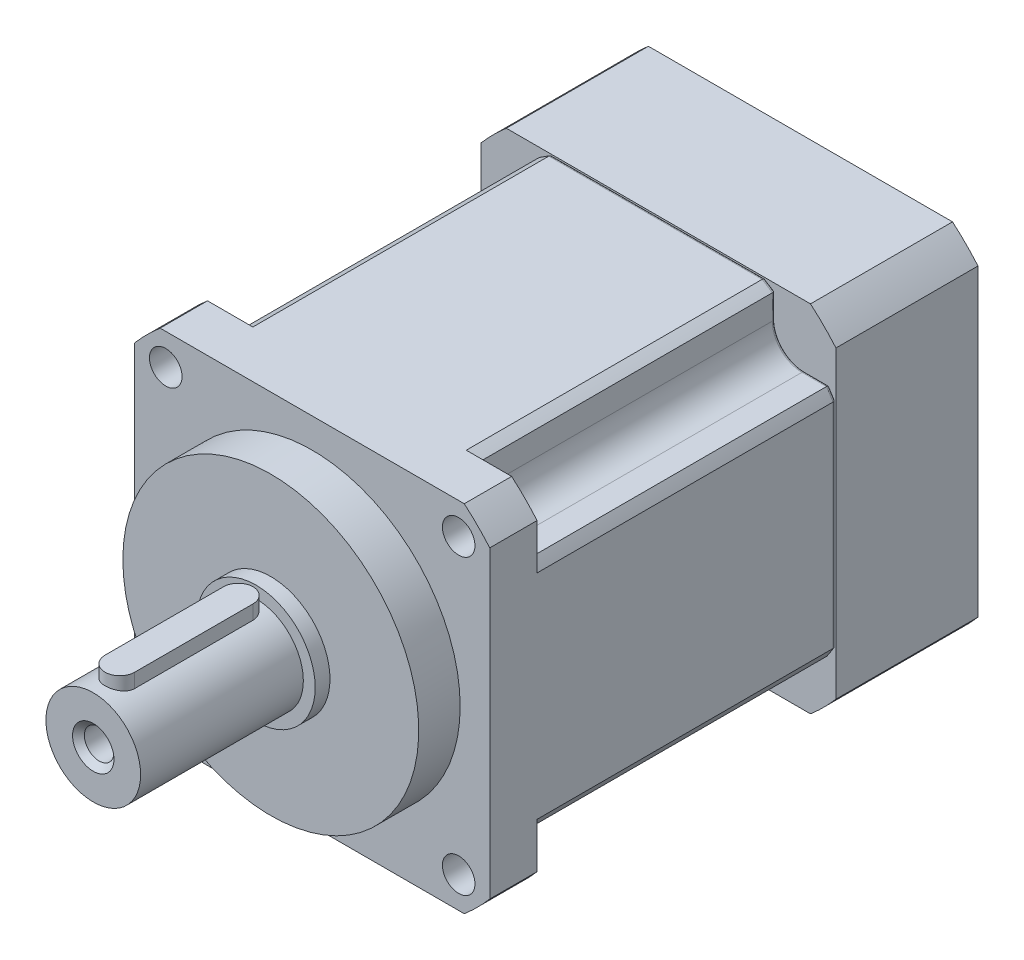
from build123d import *

# Parameters (mm, degrees)
SKETCH_1_R               = 25
EXTRUDE_2137_DEPTH       = 37
SKETCH_2_OUTSIDE_W       = 67.962
SKETCH_2_OUTSIDE_H       = 67.962
SKETCH_2_OUTSIDE_R       = 10
CUT_EXTRUDE_1_DEPTH      = 47.368092477
SKETCH_3_OUTSIDE_W       = 67.962
SKETCH_3_OUTSIDE_H       = 67.962
SKETCH_3_OUTSIDE_R       = 8
CUT_EXTRUDE_2_DEPTH      = 27.5
EXTRUDE_2_REACH          = 58.736
EXTRUDE_2_END_RADIUS     = 8
SKETCH_6_W               = 60
SKETCH_6_H               = 60
EXTRUDE_2668_DEPTH       = 58.5
CUT_EXTRUDE_8_DEPTH      = 66.956425009
PATTERN_CIRCULAR_2_COUNT = 4
CUT_EXTRUDE_6_REACH      = 74.265
SKETCH_9_R               = 2.75
PATTERN_CIRCULAR_1_COUNT = 4
SKETCH_10_OUTSIDE_W      = 87.55
SKETCH_10_OUTSIDE_H      = 87.55
SKETCH_10_OUTSIDE_R      = 39.5
CUT_EXTRUDE_7_DEPTH      = 73.265136823
FILLET_3_R               = 0.5
SKETCH_15_W              = 60
SKETCH_15_H              = 60
EXTRUDE_8537_DEPTH       = 24
SKETCH_21_OUTSIDE_W      = 91.312
SKETCH_21_OUTSIDE_H      = 91.312
SKETCH_21_OUTSIDE_R      = 39.5
CUT_EXTRUDE_10_DEPTH     = 24
SKETCH_22_R              = 25
CUT_EXTRUDE_11_DEPTH     = 5
SKETCH_30_R              = 7
CUT_EXTRUDE_15_DEPTH     = 32
PATTERN_CIRCULAR_3_COUNT = 4


with BuildPart() as part:
    # 草图1 → Extrude 2137 (new body)
    with BuildSketch(Plane.XY):
        Circle(SKETCH_1_R)
    extrude(amount=EXTRUDE_2137_DEPTH)

    # 草图2 outside → 切除-拉伸1 (cut, through all)
    with BuildSketch(Plane(origin=(0, 0, 7), x_dir=(-1, 0, 0), z_dir=(0, 0, -1))):
        Rectangle(SKETCH_2_OUTSIDE_W, SKETCH_2_OUTSIDE_H)
        Circle(SKETCH_2_OUTSIDE_R, mode=Mode.SUBTRACT)
    extrude(amount=-CUT_EXTRUDE_1_DEPTH, mode=Mode.SUBTRACT)

    # 草图3 outside → 切除-拉伸2 (cut)
    with BuildSketch(Plane.XY.offset(37)):
        Rectangle(SKETCH_3_OUTSIDE_W, SKETCH_3_OUTSIDE_H)
        Circle(SKETCH_3_OUTSIDE_R, mode=Mode.SUBTRACT)
    extrude(amount=-CUT_EXTRUDE_2_DEPTH, mode=Mode.SUBTRACT)

    # 凸台-拉伸2: up to this cylinder (the profile starts outside it)
    extrude_2_end = Plane(origin=(0, 0, 22.5), z_dir=(0, 0, 1)) * Cylinder(EXTRUDE_2_END_RADIUS, 134.472, mode=Mode.PRIVATE)
    # 草图4 → 凸台-拉伸2 (add, up to the surface)
    with BuildSketch(Plane(origin=(0, 10, 0), x_dir=(-1, 0, 0), z_dir=(0, 1, 0)), mode=Mode.PRIVATE) as extrude_2_sk1:
        with BuildLine():
            Line((-2.5, 32.5), (-2.5, 12.5))
            ThreePointArc((-2.5, 12.5), (0, 10), (2.5, 12.5))
            Line((2.5, 12.5), (2.5, 32.5))
            ThreePointArc((2.5, 32.5), (0, 35), (-2.5, 32.5))
        make_face()
    extrude_2_tool1 = extrude(extrude_2_sk1.sketch, amount=-EXTRUDE_2_REACH, mode=Mode.PRIVATE) - extrude_2_end
    add(extrude_2_tool1.solids().sort_by_distance((0, 10, 22.5))[0])

    # 草图6 → Extrude 2668 (add)
    with BuildSketch(Plane(origin=(0, 0, 0), x_dir=(-1, 0, 0), z_dir=(0, 0, -1))):
        Rectangle(SKETCH_6_W, SKETCH_6_H)
    extrude(amount=EXTRUDE_2668_DEPTH)

    # 草图7 → 切除-拉伸8 (cut, through all)
    with BuildSketch(Plane.XY.offset(-8)):
        with BuildLine():
            Line((24.748737342, 19.748737342), (28.896148072, 19.748737342))
            ThreePointArc((28.896148072, 19.748737342), (29.460643379, 18.896308944), (30, 18.027756377))
            Line((30, 18.027756377), (30, 30))
            Line((30, 30), (18.027756377, 30))
            ThreePointArc((18.027756377, 30), (18.896308944, 29.460643379), (19.748737342, 28.896148072))
            Line((19.748737342, 28.896148072), (19.748737342, 24.748737342))
            ThreePointArc((19.748737342, 24.748737342), (21.213203436, 21.213203436), (24.748737342, 19.748737342))
        make_face()
    cut_extrude_8 = extrude(amount=-CUT_EXTRUDE_8_DEPTH, mode=Mode.SUBTRACT)

    # 阵列(圆周)2: 切除-拉伸8 ×4 about axis
    pattern_circular_2_axis = Axis((0, 0, 0), (0, 0, 1))
    for i in range(1, PATTERN_CIRCULAR_2_COUNT):
        add(cut_extrude_8.rotate(pattern_circular_2_axis, i * 360 / PATTERN_CIRCULAR_2_COUNT), mode=Mode.SUBTRACT)

    # 草图9 → 切除-拉伸6 (cut, up to next)
    with BuildSketch(Plane.XY, mode=Mode.PRIVATE) as cut_extrude_6_sk1:
        with Locations((24.748737342, 24.748737342)):
            Circle(SKETCH_9_R)
    cut_extrude_6_tool1 = extrude(cut_extrude_6_sk1.sketch, amount=-CUT_EXTRUDE_6_REACH, mode=Mode.PRIVATE) & part.part
    cut_extrude_6 = cut_extrude_6_tool1.solids().sort_by_distance((24.748737, 24.748737, 0))[0]
    add(cut_extrude_6, mode=Mode.SUBTRACT)

    # 阵列(圆周)1: 切除-拉伸6 ×4 about axis
    pattern_circular_1_axis = Axis((0, 0, 0), (0, 0, 1))
    for i in range(1, PATTERN_CIRCULAR_1_COUNT):
        add(cut_extrude_6.rotate(pattern_circular_1_axis, i * 360 / PATTERN_CIRCULAR_1_COUNT), mode=Mode.SUBTRACT)

    # 草图10 outside → 切除-拉伸7 (cut, through all)
    with BuildSketch(Plane.XY):
        Rectangle(SKETCH_10_OUTSIDE_W, SKETCH_10_OUTSIDE_H)
        Circle(SKETCH_10_OUTSIDE_R, mode=Mode.SUBTRACT)
    extrude(amount=-CUT_EXTRUDE_7_DEPTH, mode=Mode.SUBTRACT)

    # 圆角3
    fillet_3_edges = [part.edges().sort_by_distance(p)[0] for p in [
        (-30, 0, -58.5),
        (-18.896308944, -29.460643379, -58.5),
        (-29.460643379, -18.896308944, -58.5),
        (-26.822442707, -19.748737342, -58.5),
        (-21.213203436, -21.213203436, -58.5),
        (-19.748737342, -26.822442707, -58.5),
        (0, 30, -58.5),
        (-29.460643379, 18.896308944, -58.5),
        (-18.896308944, 29.460643379, -58.5),
        (-19.748737342, 26.822442707, -58.5),
        (-21.213203436, 21.213203436, -58.5),
        (-26.822442707, 19.748737342, -58.5),
        (30, 0, -58.5),
        (18.896308944, 29.460643379, -58.5),
        (29.460643379, 18.896308944, -58.5),
        (26.822442707, 19.748737342, -58.5),
        (21.213203436, 21.213203436, -58.5),
        (19.748737342, 26.822442707, -58.5),
        (0, -30, -58.5),
        (29.460643379, -18.896308944, -58.5),
        (18.896308944, -29.460643379, -58.5),
        (19.748737342, -26.822442707, -58.5),
        (21.213203436, -21.213203436, -58.5),
        (26.822442707, -19.748737342, -58.5),
    ]]
    fillet(fillet_3_edges, radius=FILLET_3_R)

    # 草图15 → Extrude 8537 (add)
    with BuildSketch(Plane(origin=(0, 0, -58.5), x_dir=(-1, 0, 0), z_dir=(0, 0, -1))):
        Rectangle(SKETCH_15_W, SKETCH_15_H)
    extrude(amount=EXTRUDE_8537_DEPTH)

    # 草图21 outside → 切除-拉伸10 (cut)
    with BuildSketch(Plane(origin=(0, 0, -82.5), x_dir=(-1, 0, 0), z_dir=(0, 0, -1))):
        Rectangle(SKETCH_21_OUTSIDE_W, SKETCH_21_OUTSIDE_H)
        Circle(SKETCH_21_OUTSIDE_R, mode=Mode.SUBTRACT)
    extrude(amount=-CUT_EXTRUDE_10_DEPTH, mode=Mode.SUBTRACT)

    # 草图22 → 切除-拉伸11 (cut)
    with BuildSketch(Plane(origin=(0, 0, -82.5), x_dir=(-1, 0, 0), z_dir=(0, 0, -1))):
        Circle(SKETCH_22_R)
    extrude(amount=-CUT_EXTRUDE_11_DEPTH, mode=Mode.SUBTRACT)

    # 草图30 → 切除-拉伸15 (cut)
    with BuildSketch(Plane(origin=(0, 0, -82.5), x_dir=(-1, 0, 0), z_dir=(0, 0, -1))):
        Circle(SKETCH_30_R)
    extrude(amount=-CUT_EXTRUDE_15_DEPTH, mode=Mode.SUBTRACT)

    # 草图31 → M5 螺纹孔1 (revolve, cut)
    with BuildSketch(Plane(origin=(0, 0, 37), x_dir=(0, -1, 0), z_dir=(1, 0, 0))):
        Polygon((0, 0), (0, 15.201721238), (2, 14), (2, 12), (2.5, 12), (2.5, 1), (3.5, 0), align=None)
    revolve(axis=Axis((0, 0, 43.35), (0, 0, -1)), mode=Mode.SUBTRACT)

    # 草图34 → M5 螺纹孔2 (revolve, cut)
    with BuildSketch(Plane(origin=(-24.748737342, 24.748737342, -82.5), x_dir=(0, 1, 0), z_dir=(1, 0, 0))):
        Polygon((0, 0), (0, 13.201721238), (2, 12), (2, 10), (2.5, 10), (2.5, 0), align=None)
    hole_wizard_m5_2 = revolve(axis=Axis((-24.748737342, 24.748737342, -88.85), (0, 0, 1)), mode=Mode.SUBTRACT)

    # 阵列(圆周)3: M5 螺纹孔2 ×4 about axis
    pattern_circular_3_axis = Axis((0, 0, 0), (0, 0, 1))
    for i in range(1, PATTERN_CIRCULAR_3_COUNT):
        add(hole_wizard_m5_2.rotate(pattern_circular_3_axis, i * 360 / PATTERN_CIRCULAR_3_COUNT), mode=Mode.SUBTRACT)


solid = part.part
